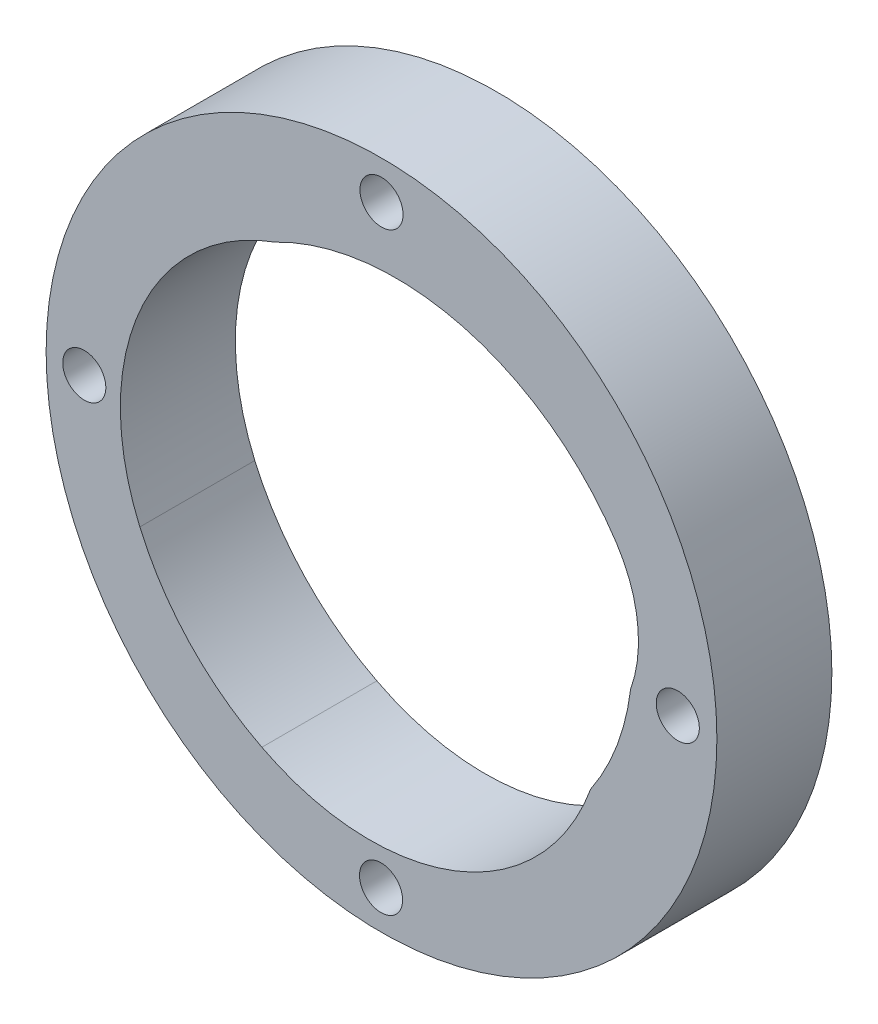
SolidWorks part; units mm, degrees
ref_plane "前视基准面" through (0, 0, 0) normal (0, 0, 1) x (1, 0, 0)
ref_plane "上视基准面" through (0, 0, 0) normal (0, 1, 0) x (1, 0, 0)
ref_plane "右视基准面" through (0, 0, 0) normal (1, 0, 0) x (0, 0, -1)
sketch "草图2" plane through (0, 0, 0) normal (0, 0, 1) x (1, 0, 0)
  line L0 (-47.2422, 0) -> (38.4512, 0) construction
  line L1 (0, 37.0723) -> (0, -43.8189) construction
  line L2 (0, 0) -> (21.3756, 41.952) construction
  line L3 (0, 0) -> (36.5935, 18.6453) construction
  line L4 (0, 0) -> (-17.0778, 33.5171) construction
  line L5 (0, 0) -> (35.1811, -17.9257) construction
  line L6 (0, 0) -> (14.7837, -29.0147) construction
  line L7 (0, 0) -> (-32.4092, -16.5133) construction
  line L8 (0, 0) -> (-17.8043, -34.943) construction
  arc A0 (-25.2211, -10.9612) -> (-9.3897, -25.8473) centre (0, 0) ccw
  arc A1 (-25.2211, -10.9612) -> (-11.1228, 21.8297) centre (-2.7514, -1.1958) cw
  arc A2 (-11.1228, 21.8297) -> (24.5027, 12.4847) centre (1.5079, -2.5981) cw
  arc A3 (24.5027, 12.4847) -> (26, 0) centre (12.6888, 4.7357) cw
  arc A4 (26, 0) -> (21.8297, -11.1228) centre (0.8873, 3.0725) cw
  arc A5 (-12.4847, -24.5027) -> (21.8297, -11.1228) centre (-1.1979, -2.7574) ccw
  circle A6 centre (0, 0) radius 35
  point P7 (-11.1228, 21.8297)
  point P19 (26, 0)
  point P22 (21.8297, -11.1228)
  dimension "D1" = 55
  dimension "D10" = 26
  dimension "D11" = 54
  dimension "D2" = 27
  dimension "D3" = 36
  dimension "D4" = 27
  dimension "D5" = 27
  dimension "D6" = 36
  dimension "D7" = 27
  dimension "D8" = 27
  dimension "D9" = 24.5
  dimension "D12" = 24.5
extrude "凸台-拉伸1" add sketch "草图2" along normal blind 12 contours A6 A5 A0 A1 A2 A3 A4
sketch "草图3" plane through (0, 0, 12) normal (0, 0, 1) x (1, 0, 0)
  line L0 (-40.1044, 0) -> (44.8458, 0) construction
  line L1 (0, 37.2892) -> (0, -40.2526) construction
  circle A0 centre (0, 0) radius 31 construction
  circle A1 centre (0, 31) radius 2.25
  circle A2 centre (30.9179, 0.0494) radius 2.25
  circle A3 centre (-0.0474, -30.9786) radius 2.25
  circle A4 centre (-31.0167, -0.1482) radius 2.25
extrude "切除-拉伸1" cut sketch "草图3" against normal through all
